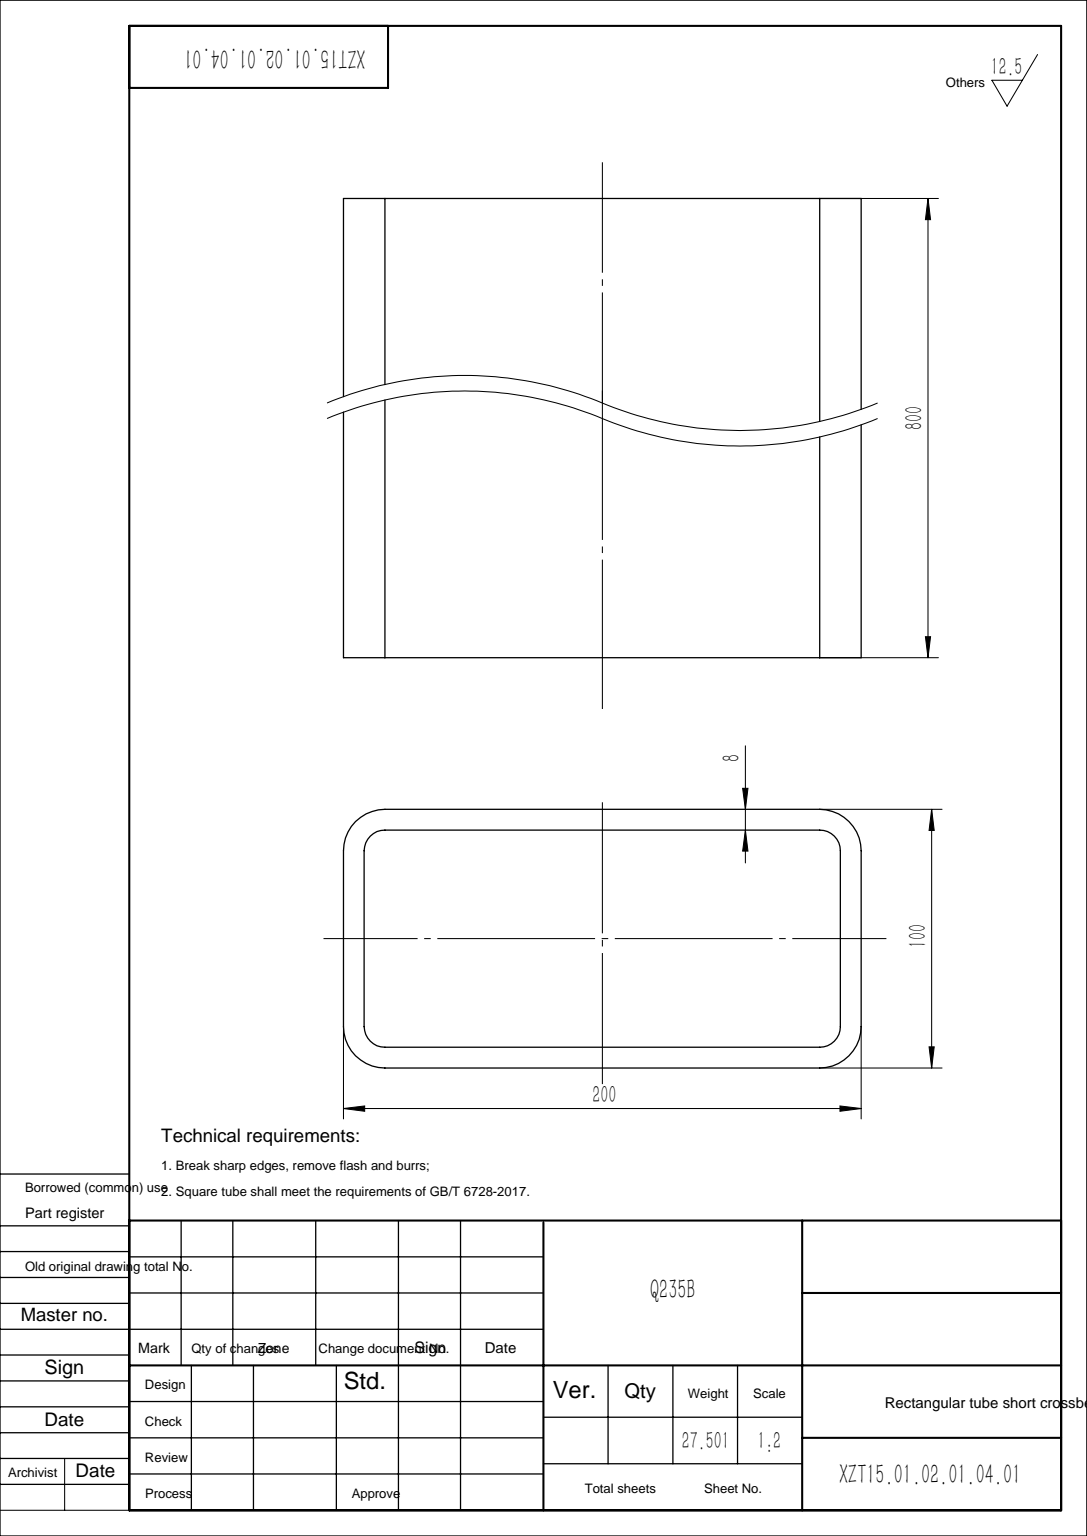
from build123d import *

# Parameters (mm, degrees)
GB_T_6728_2002_RECTANGULAR_HOLLOW_SECTIO_DEPTH = 800


with BuildPart() as part:
    # Sketch12 → GB/T 6728-2002 rectangular hollow section 200X100X8(2) (new body)
    with BuildSketch(Plane.ZX):
        with BuildLine():
            Line((-34, -100), (34, -100))
            ThreePointArc((34, -100), (45.313708499, -95.313708499), (50, -84))
            Line((50, -84), (50, 84))
            ThreePointArc((50, 84), (45.313708499, 95.313708499), (34, 100))
            Line((34, 100), (-34, 100))
            ThreePointArc((-34, 100), (-45.313708499, 95.313708499), (-50, 84))
            Line((-50, 84), (-50, -84))
            ThreePointArc((-50, -84), (-45.313708499, -95.313708499), (-34, -100))
        make_face()
        with BuildLine():
            Line((-34, -92), (34, -92))
            ThreePointArc((34, -92), (39.656854249, -89.656854249), (42, -84))
            Line((42, -84), (42, 84))
            ThreePointArc((42, 84), (39.656854249, 89.656854249), (34, 92))
            Line((34, 92), (-34, 92))
            ThreePointArc((-34, 92), (-39.656854249, 89.656854249), (-42, 84))
            Line((-42, 84), (-42, -84))
            ThreePointArc((-42, -84), (-39.656854249, -89.656854249), (-34, -92))
        make_face(mode=Mode.SUBTRACT)
    extrude(amount=GB_T_6728_2002_RECTANGULAR_HOLLOW_SECTIO_DEPTH)


solid = part.part
